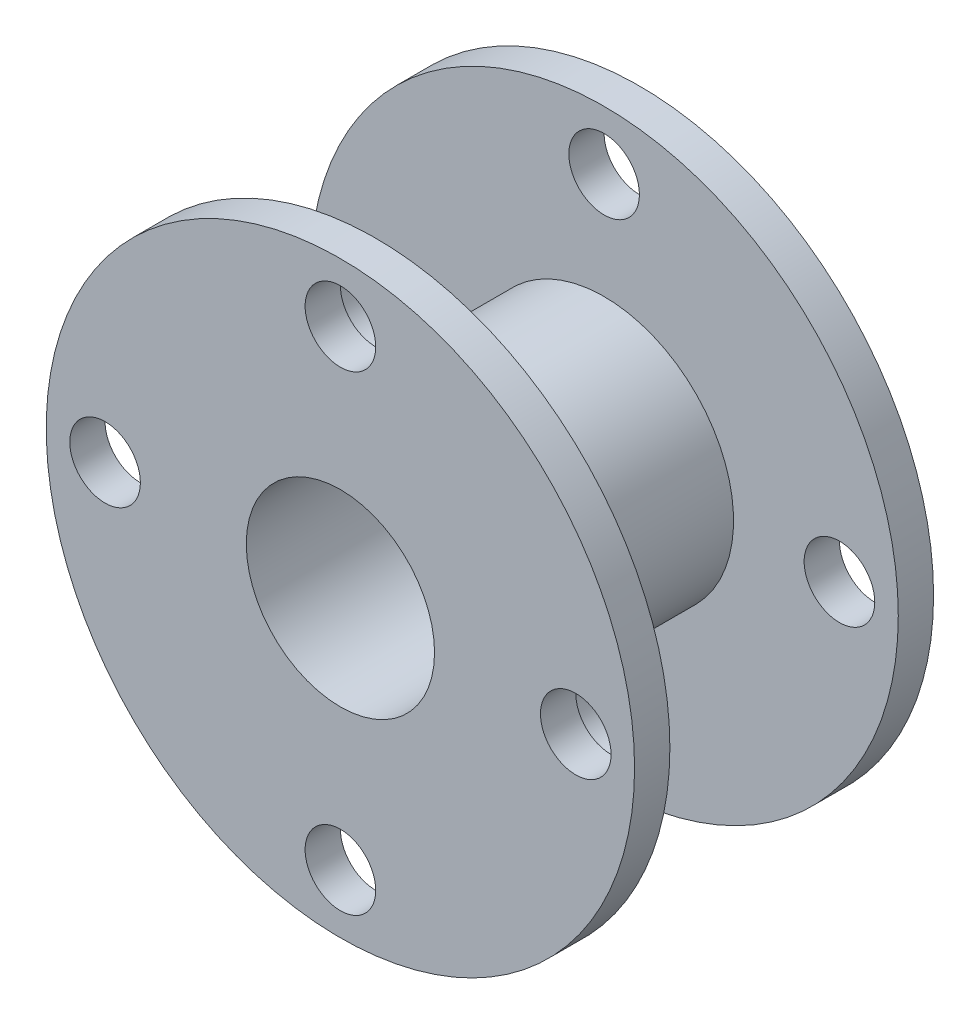
from build123d import *

# Parameters (mm, degrees)
SKETCH_1_R        = 11
SKETCH_1_R_2      = 8
EXTRUDE_1_DEPTH   = 12.705
EXTRUDE_START     = -3
SKETCH_2_R        = 25
SKETCH_2_R_2      = 8
SKETCH_2_R_3      = 3
EXTRUDE_1_2_DEPTH = 3


with BuildPart() as part:
    # 草图1 → Extrude 1 (new, symmetric)
    with BuildSketch(Plane.XY):
        Circle(SKETCH_1_R)
        Circle(SKETCH_1_R_2, mode=Mode.SUBTRACT)
    extrude(amount=EXTRUDE_1_DEPTH, both=True)

    # 草图2 → Extrude 1 2 (add)
    with BuildSketch(Plane.XY.offset(12.705).offset(EXTRUDE_START)):
        Circle(SKETCH_2_R)
        Circle(SKETCH_2_R_2, mode=Mode.SUBTRACT)
        with Locations((0, 20)):
            Circle(SKETCH_2_R_3, mode=Mode.SUBTRACT)
        with Locations((20, 0)):
            Circle(SKETCH_2_R_3, mode=Mode.SUBTRACT)
        with Locations((0, -20)):
            Circle(SKETCH_2_R_3, mode=Mode.SUBTRACT)
        with Locations((-20, 0)):
            Circle(SKETCH_2_R_3, mode=Mode.SUBTRACT)
    extrude_1_2 = extrude(amount=EXTRUDE_1_2_DEPTH)

    # 镜向1: Extrude 1 2 across plane
    add(extrude_1_2.mirror(Plane.XY))


solid = part.part
